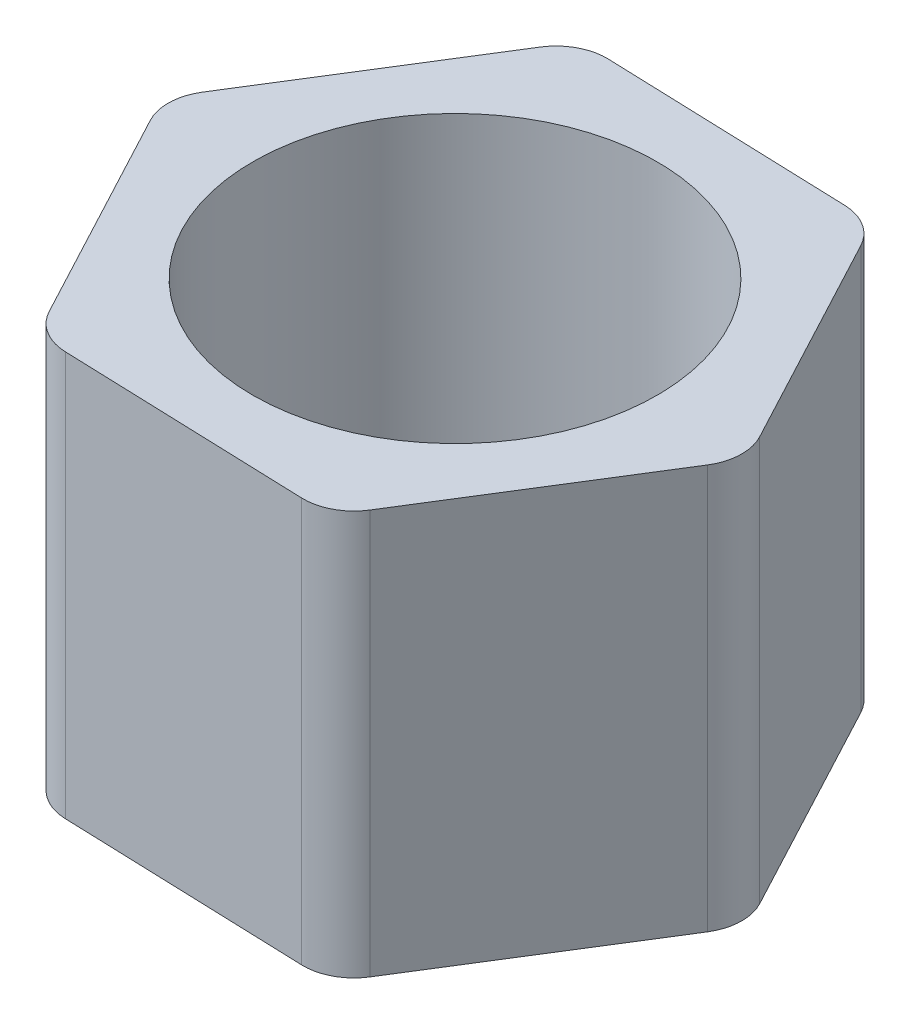
from build123d import *

# Parameters (mm, degrees)
SKETCH1_R           = 8
BOSS_EXTRUDE1_DEPTH = 16
FILLET1_R           = 2
FILLET2_R           = 2


with BuildPart() as part:
    # Sketch1 → Boss-Extrude1 (new body)
    with BuildSketch(Plane(origin=(0, 0, 0), x_dir=(1, 0, 0), z_dir=(0, 1, 0))):
        Polygon((5.636967427, -10.593611199), (11.992820129, -0.415048607), (6.355852702, 10.178562591), (-5.636967427, 10.593611199), (-11.992820129, 0.415048607), (-6.355852702, -10.178562591), align=None)
        with Locations(Location((0, 0, 0), (0, 0, 270))):
            Circle(SKETCH1_R, mode=Mode.SUBTRACT)
    extrude(amount=BOSS_EXTRUDE1_DEPTH)

    # Fillet1
    fillet1_edges = [part.edges().sort_by_distance(p)[0] for p in [
        (5.636967427, 8, 10.593611199),
    ]]
    fillet(fillet1_edges, radius=FILLET1_R)

    # Fillet2
    fillet2_edges = [part.edges().sort_by_distance(p)[0] for p in [
        (-6.355852702, 8, 10.178562591),
        (-11.992820129, 8, -0.415048607),
        (-5.636967427, 8, -10.593611199),
        (6.355852702, 8, -10.178562591),
        (11.992820129, 8, 0.415048607),
    ]]
    fillet(fillet2_edges, radius=FILLET2_R)


solid = part.part
